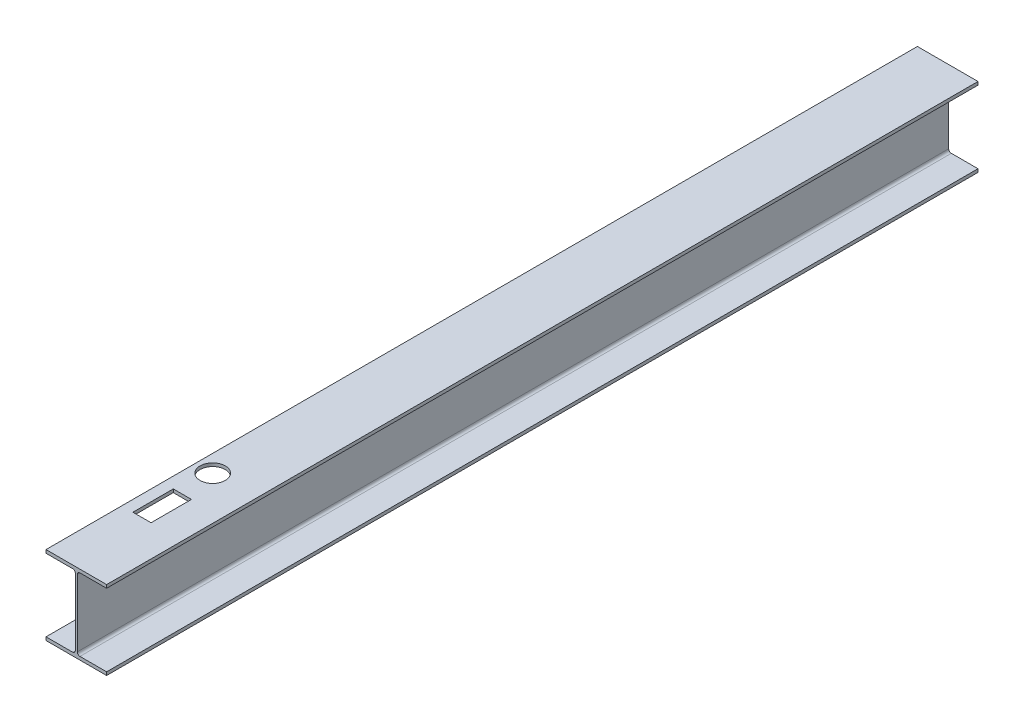
SolidWorks part; units mm, degrees
material "Q235"
ref_plane "Front Plane" through (0, 0, 0) normal (0, 0, 1) x (1, 0, 0)
ref_plane "Top Plane" through (0, 0, 0) normal (0, 1, 0) x (1, 0, 0)
ref_plane "Right Plane" through (0, 0, 0) normal (1, 0, 0) x (0, 0, -1)
sketch "Sketch1" plane through (0, 0, 0) normal (0, 0, 1) x (1, 0, 0)
  line L0 (0, 0) -> (300, 0)
  line L1 (300, 0) -> (300, 16)
  line L2 (300, 16) -> (168, 16)
  line L3 (155, 29) -> (155, 361)
  line L4 (168, 374) -> (300, 374)
  line L5 (300, 374) -> (300, 390)
  line L6 (300, 390) -> (0, 390)
  line L7 (0, 390) -> (0, 374)
  line L8 (0, 374) -> (132, 374)
  line L9 (145, 361) -> (145, 29)
  line L10 (132, 16) -> (0, 16)
  line L11 (0, 16) -> (0, 0)
  line L12 (150, 390) -> (150, 0) construction
  arc A0 (168, 16) -> (155, 29) centre (168, 29) cw
  arc A1 (145, 29) -> (132, 16) centre (132, 29) cw
  arc A2 (155, 361) -> (168, 374) centre (168, 361) cw
  arc A3 (132, 374) -> (145, 361) centre (132, 361) cw
  point P21 (155, 374)
  dimension "D7" = 13
  dimension "D1" = 390
  dimension "D2" = 300
  dimension "D3" = 10
  dimension "D4" = 5
  dimension "D5" = 16
  dimension "D6" = 16
extrude "Boss-Extrude1" add sketch "Sketch1" along normal blind 4313
sketch "Sketch2" plane through (0, 390, 0) normal (0, 1, 0) x (1, 0, 0)
  line L1 (145, -3738) -> (55, -3738)
  line L2 (145, -3738) -> (145, -3938)
  line L3 (145, -3938) -> (55, -3938)
  line L4 (55, -3738) -> (55, -3938)
  line L5 (0, -4313) -> (0, 0) construction
  line L6 (300, -4313) -> (0, -4313) construction
  circle A0 centre (85, -3573) radius 62.5
  dimension "D1" = 125
  dimension "D2" = 85
  dimension "D3" = 375
  dimension "D6" = 365
  dimension "D4" = 200
  dimension "D5" = 90
  dimension "D7" = 55
extrude "Cut-Extrude1" cut sketch "Sketch2" against normal blind 30
sketch "Sketch3" plane through (145, 0, 0) normal (-1, 0, 0) x (0, 0, 1)
  line L0 (4313, 361) -> (4313, 29) construction
  line L1 (3938, 390) -> (3738, 390) construction
  circle A0 centre (3838, 315) radius 25.5
  dimension "D1" = 51
  dimension "D2" = 475
  dimension "D3" = 75
extrude "Cut-Extrude2" cut sketch "Sketch3" against normal up to next
